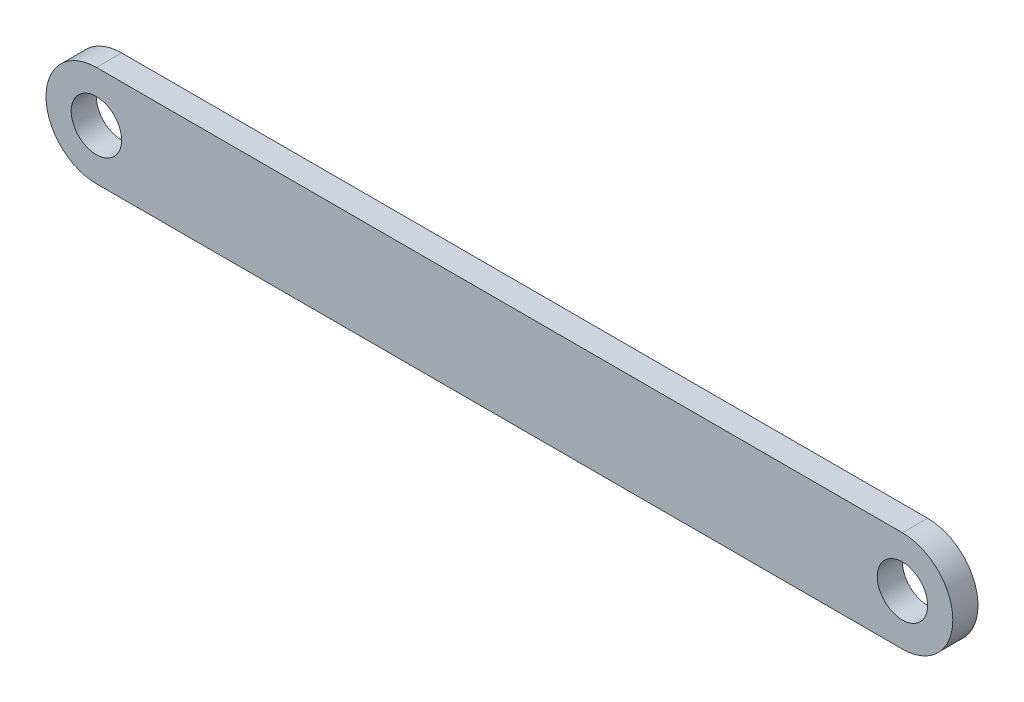
from build123d import *

# Parameters (mm, degrees)
SKETCH1_R           = 2
BOSS_EXTRUDE1_DEPTH = 2


with BuildPart() as part:
    # Sketch1 → Boss-Extrude1 (new body)
    with BuildSketch(Plane.XY):
        with BuildLine():
            Line((0, 4), (64, 4))
            ThreePointArc((64, 4), (68, 0), (64, -4))
            Line((64, -4), (0, -4))
            ThreePointArc((0, -4), (-4, 0), (0, 4))
        make_face()
        Circle(SKETCH1_R, mode=Mode.SUBTRACT)
        with Locations((64, 0)):
            Circle(SKETCH1_R, mode=Mode.SUBTRACT)
    extrude(amount=BOSS_EXTRUDE1_DEPTH)


solid = part.part
